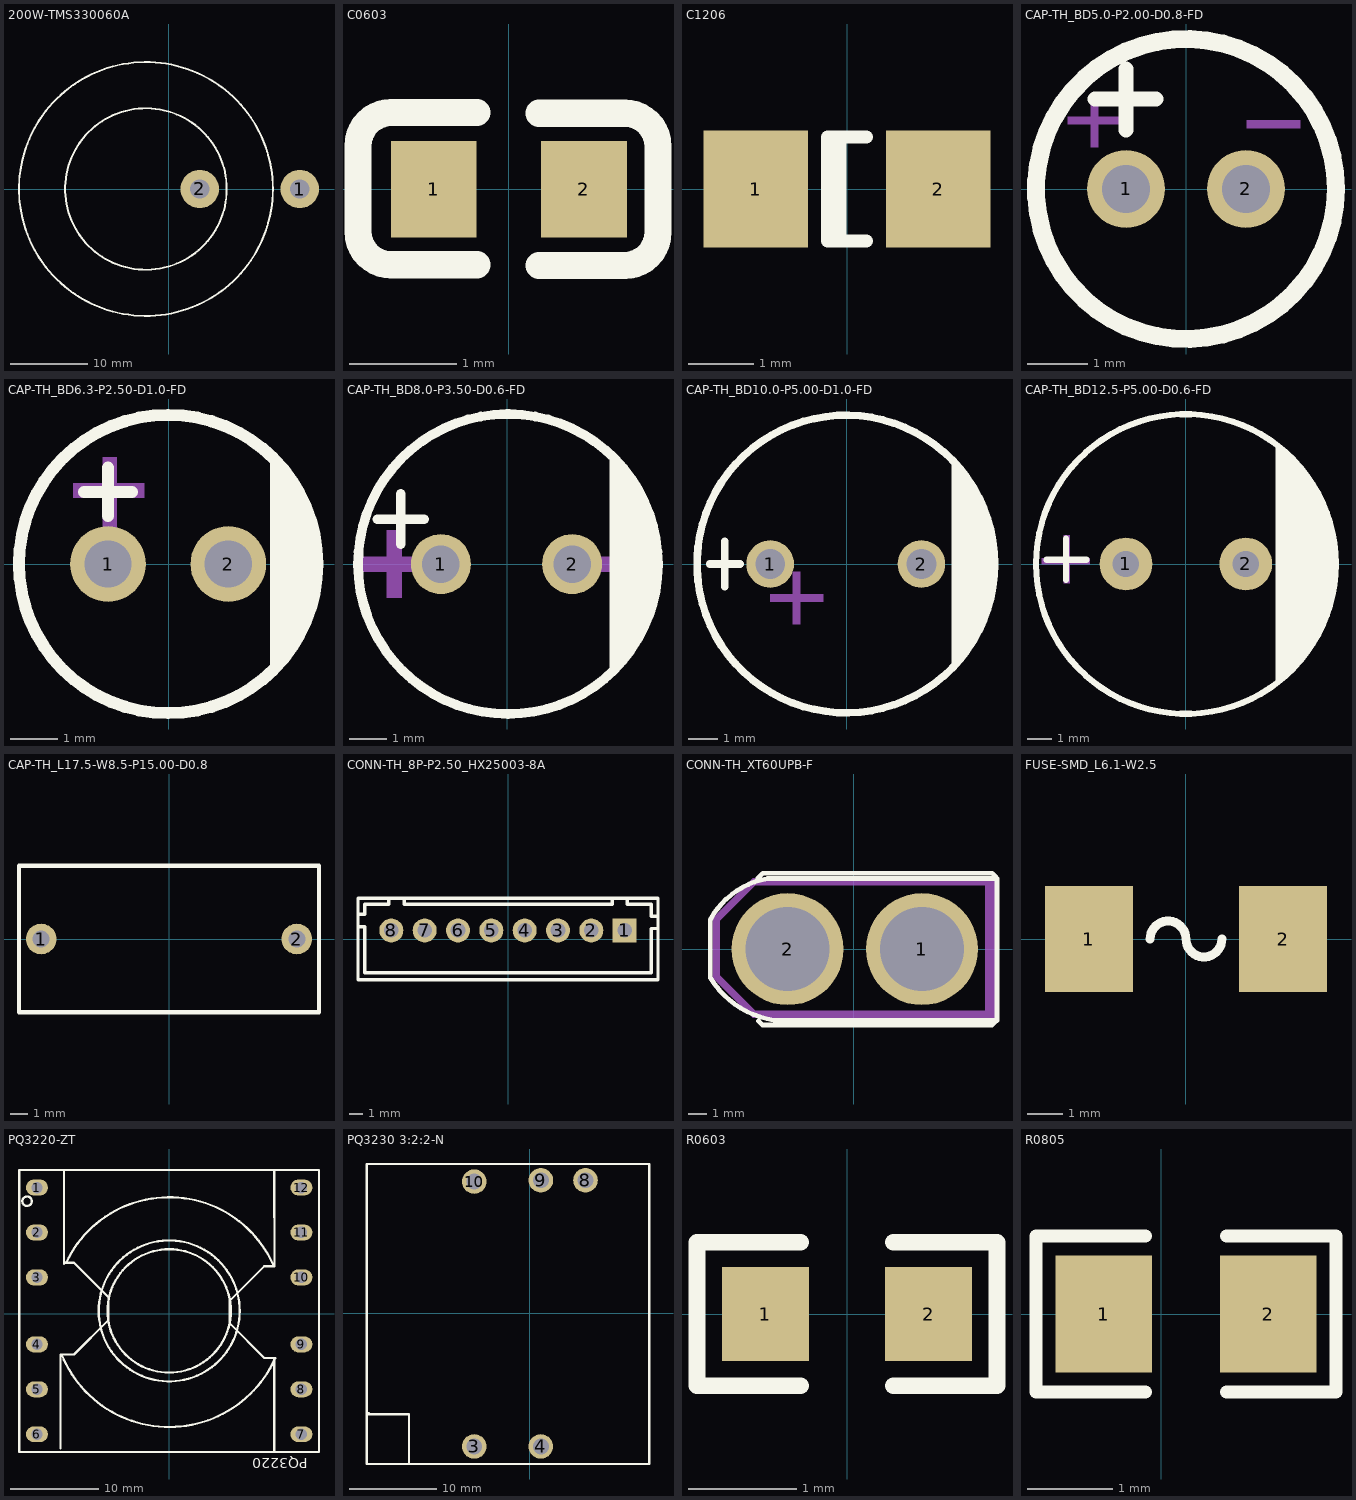
[diagram p0: the footprints below, top view; thin cyan lines are the x and y axes]
# Altium footprint library MISC84449-2.PcbLib: 30 footprints (part 1 of 2)
Each footprint in its own frame and in the unit in brackets; x right, y up, seen from the top. Pads: shape width x height; smd on the part's side, far side on the other; paste and mask are expansions set on the pad; w line width, h text height; cw(c..) or ccw(c..) is an arc to the next point about the centre after c.

## 200W-TMS330060A [mm]
pads (2):
  round 5 hole 2.5: 1(17,0) 2(4,0)
Top Overlay:
  circle w0.254: c-3,0 r16.5
  circle w0.254: c-3,0 r10.5

## C0603 [mm]
pads (2):
  rect 0.8x0.9 smd: 1(-0.7,0) 2(0.7,0)
Top Overlay:
  lines w0.254: -0.296,-0.704 -1.096,-0.704 cw(c-1.096,-0.394) -1.406,-0.394 -1.405,0.406 cw(c-1.096,0.406) -1.096,0.715 -0.296,0.715 ; 0.28,-0.71 1.08,-0.71 ccw(c1.08,-0.4) 1.39,-0.4 1.39,0.4 ccw(c1.08,0.4) 1.08,0.71 0.28,0.71

## C1206 [mm] "Chip Capacitor; Body 3.2 x 1.6 mm (LxW typ)"
height 1.35
pads (2):
  rect 1.6x1.8 smd: 1(-1.4,0) 2(1.4,0)
Top Overlay:
  lines w0.2: -0.11,-0.8 -0.11,0.8 ; 0.3,-0.8 -0.3,-0.8 -0.3,0.8 0.3,0.8

## CAP-TH_BD5.0-P2.00-D0.8-FD [mm]
pads (2):
  round 1.3 hole 0.8: 1(-1,0) 2(1,0)
Top Overlay:
  circle w0.3: c0,0 r2.5
  lines w0.254: -1.516,1.5 -0.5,1.5 ; -1,0.984 -1,2
Mechanical 15:
  region: 1.016,1.143 1.905,1.143 1.905,1.016 1.016,1.016
  region: -1.588,0.699 -1.588,1.587 -1.461,1.587 -1.46,0.699
  region: -1.969,1.206 -1.08,1.206 -1.08,1.079 -1.969,1.079

## CAP-TH_BD6.3-P2.50-D1.0-FD [mm]
pads (2):
  round 1.6 hole 1: 1(-1.28,0) 2(1.26,0)
Top Overlay:
  circle w0.254: c-0.01,0 r3.15
  region: 2.15,2.287 2.27,2.184 2.585,1.816 2.838,1.402 3.023,0.955 3.136,0.483 3.175,0 3.136,-0.483 3.023,-0.955 2.838,-1.402 2.585,-1.816 2.27,-2.184 2.15,-2.287 2.149,-2.286
  lines w0.254: -1.788,1.524 -0.772,1.524 ; -1.28,1.016 -1.28,2.032
Mechanical 15:
  region: -2.01,1.7 -0.51,1.7 -0.51,1.4 -2.01,1.4
  region: -1.391,0.752 -1.391,2.252 -1.091,2.252 -1.091,0.752

## CAP-TH_BD8.0-P3.50-D0.6-FD [mm]
pads (2):
  round 1.6 hole 1: 1(-1.769,-0.001) 2(1.731,-0.001)
Top Overlay:
  region: 2.734,-3.003 3.039,-2.654 3.356,-2.18 3.608,-1.669 3.792,-1.129 3.903,-0.57 3.94,-0.001 3.903,0.568 3.792,1.128 3.608,1.668 3.356,2.179 3.039,2.653 2.734,3.002 2.731,2.999
  lines w0.254: -3.464,1.199 -2.219,1.199 ; -2.841,0.526 -2.841,1.873 ; -0.017,4 ccw(c0.019,0) 0.055,4
Mechanical 15:
  region: -3.219,-0.901 -2.819,-0.901 -2.819,0.899 -3.219,0.899
  region: -3.919,0.199 -3.919,-0.201 -2.119,-0.201 -2.119,0.199
  region: 2.081,0.199 2.081,-0.201 3.881,-0.201 3.881,0.199

## CAP-TH_BD10.0-P5.00-D1.0-FD [mm]
pads (2):
  round 1.6 hole 1: 1(-2.578,0) 2(2.502,0)
Top Overlay:
  circle w0.254: c-0.038,0 r5
  region: 3.518,3.556 3.518,-3.556 4.28,-2.54 4.788,-1.016 5.042,0.508 4.788,1.524
  lines w0.254: -4.61,0 -3.594,0 ; -4.102,-0.762 -4.102,0.762
Mechanical 15:
  region: -1.816,-2.032 -1.562,-2.032 -1.562,-0.254 -1.816,-0.254
  region: -2.578,-1.016 -0.8,-1.016 -0.8,-1.27 -2.578,-1.27

## CAP-TH_BD12.5-P5.00-D0.6-FD [mm]
pads (2):
  round 2.2 hole 1.1: 1(-2.5,0) 2(2.5,0)
Top Overlay:
  circle w0.254: c0,0 r6.25
  region: 3.75,5 3.75,-5 4.482,-4.268 4.489,-4.274 4.941,-3.769 5.333,-3.216 5.661,-2.623 5.92,-1.997 6.108,-1.345 6.221,-0.677 6.259,0 6.221,0.677 6.108,1.345 5.92,1.997 5.661,2.623 5.333,3.216 4.941,3.769 4.489,4.274 4.482,4.268
  lines w0.254: -5.817,0.178 -4.14,0.178 ; -5.004,-0.66 -5.004,1.067
Mechanical 15:
  region: -5.092,-0.811 -5.092,1.189 -4.842,1.189 -4.842,-0.811
  region: -6,0.25 -4,0.25 -4,0 -6,0

## CAP-TH_L17.5-W8.5-P15.00-D0.8 [mm]
pads (2):
  round 1.8 hole 1: 1(-7.5,0) 2(7.5,0)
Top Overlay:
  lines w0.254: -8.8,-4.3 8.8,-4.3 8.8,4.3 -8.8,4.3 -8.8,-4.3

## CONN-TH_8P-P2.50_HX25003-8A [mm]
pads (8):
  rect 1.8x1.8 hole 1.1: 1(8.75,0.646)
  round 1.8 hole 1.1: 2(6.25,0.646) 3(3.75,0.646) 4(1.25,0.646) 5(-1.25,0.646) 6(-3.75,0.646) 7(-6.25,0.646) 8(-8.75,0.646)
Top Overlay:
  lines w0.254: -11.25,0.915 -10.75,0.915 -10.75,-2.521 10.749,-2.521 10.749,0.786 11.249,0.786 ; -11.25,1.845 -10.75,1.845 -10.75,2.604 -8.944,2.604 -8.944,3.054 ; -7.8,2.604 7.8,2.604 ; -7.793,2.601 -7.793,3.05 ; 7.807,2.601 7.807,3.05 ; 8.943,2.604 10.749,2.604 10.749,1.715 11.249,1.715 ; 8.95,2.602 8.95,3.05 ; -11.25,-3.054 11.25,-3.054 11.25,3.046 -11.25,3.046 -11.25,-3.054

## CONN-TH_XT60UPB-F [mm]
pads (2):
  round 6 hole 4.5: 1(3.663,0) 2(-3.536,0)
Top Overlay:
  lines w0.254: -7.683,-1.524 -7.683,1.576 cw(c-3.873,-0.482) -4.625,3.783 7.683,3.783 7.683,-3.819 ; -7.668,-1.548 ccw(c-3.507,1.016) -4.283,-3.81 7.658,-3.81 ; -5.119,3.819 -4.874,4.064 -4.827,4.064 7.419,4.064 7.638,3.844 ; -5.099,-3.844 -4.88,-4.064 7.365,-4.064 7.413,-4.064 7.658,-3.819
Mechanical 15:
  region: -5.397,3.81 -7.556,1.651 -7.303,1.397 -5.143,3.556
  region: -7.556,-1.524 -5.397,-3.683 -5.143,-3.429 -7.302,-1.27
  region: -7.556,1.651 -7.556,-1.524 -7.175,-1.524 -7.175,1.651
  region: -5.397,3.81 7.556,3.81 7.556,3.429 -5.271,3.429
  region: -5.397,-3.683 -5.397,-3.302 7.556,-3.302 7.556,-3.683
  region: 7.556,3.429 7.556,-3.302 7.049,-3.302 7.049,3.429

## FUSE-SMD_L6.1-W2.5 [mm]
pads (2):
  rect 2.5x3 smd: 1(-2.75,0) 2(2.75,0)
Top Overlay:
  lines w0.254: -1.016,0 cw(c-0.508,0) 0,0 ccw(c0.508,0) 1.016,0

## PQ3220-ZT [mm]
pads (12):
  oval 2.5x1.8 hole 1.3: 1(-14.98,14.318) 2(-14.98,9.218) 3(-14.98,4.119) 4(-14.98,-3.481) 5(-14.98,-8.581) 6(-14.98,-13.681) 7(15.02,-13.682) 8(15.02,-8.581) 9(15.02,-3.481) 10(15.02,4.119) 11(15.02,9.218) 12(15.02,14.318)
Top Overlay:
  circle w0.254: c0.02,0.319 r7
  circle w0.254: c0.02,0.319 r8
  circle w0.254: c-16.109,12.765 r0.539
  lines w0.254: -17.02,16.318 17.02,16.318 ; -16.98,-15.681 -16.98,16.318 ; -16.957,-15.681 17.02,-15.681 ; -12.299,-15.302 -12.299,-4.637 ; -11.918,5.78 -10.787,5.78 -6.85,1.843 -6.85,-0.697 -10.787,-4.634 -12.184,-4.634 ccw(c0.02,0.319) 12.044,-5.059 ; -11.903,5.653 -11.903,16.318 ; -11.647,5.83 cw(c0.02,0.319) 11.788,5.614 ; 11.946,-15.681 11.946,-5.015 10.815,-5.015 6.878,-1.078 6.878,1.462 10.815,5.399 11.958,5.399 11.946,16.318 ; 17.02,-15.687 17.02,16.315
  text "PQ3220" at 15.748,-16.383 h1.14

## PQ3230 3:2:2-N [mm]
pads (5):
  round 2.8 hole 1.8: 3(-6.342,-15.17) 4(1.258,-15.17) 8(6.342,15.17) 9(1.262,15.17) 10(-6.342,15.03)
Top Overlay:
  lines w0.254: -18.364,-11.372 -18.364,-11.499 -13.787,-11.499 -13.787,-17.168 -12.141,-17.168 ; -18.59,-17.169 13.61,-17.169 13.61,17.031 -18.59,17.031 -18.59,-17.169

## R0603 [mm]
pads (2):
  rect 0.806x0.864 smd: 1(-0.753,0) 2(0.753,0)
Top Overlay:
  lines w0.152: -0.426,-0.661 -1.385,-0.661 -1.385,0.661 -0.426,0.661 ; 0.426,-0.661 1.385,-0.661 1.385,0.661 0.426,0.661
Top Paste:
  region: -0.355,0.4 -0.355,0.172 -0.735,0.172 -0.735,-0.158 -0.355,-0.158 -0.355,-0.4 -0.405,-0.45 -1.195,-0.45 -1.245,-0.4 -1.245,0.4 -1.195,0.45 -0.405,0.45
  region: 1.195,0.45 0.395,0.45 0.345,0.4 0.345,0.172 0.715,0.172 0.715,-0.158 0.345,-0.158 0.345,-0.4 0.395,-0.45 1.195,-0.45 1.245,-0.4 1.245,0.4

## R0805 [mm]
pads (2):
  rect 1.133x1.377 smd: 1(-0.678,0) 2(1.254,0)
Top Overlay:
  lines w0.152: -0.188,-0.917 -1.473,-0.917 -1.473,0.917 -0.188,0.917 ; 0.764,-0.917 2.049,-0.917 2.049,0.917 0.764,0.917
Top Paste:
  region: 0.738,-0.64 0.738,-0.22 1.183,-0.22 1.183,0.23 0.743,0.23 0.738,0.64 0.788,0.69 1.938,0.69 1.988,0.64 1.988,-0.64 1.938,-0.69 0.788,-0.69
  region: -1.412,-0.64 -1.412,0.64 -1.362,0.69 -0.212,0.69 -0.162,0.64 -0.157,0.23 -0.607,0.23 -0.607,-0.22 -0.167,-0.22 -0.162,-0.64 -0.212,-0.69 -1.362,-0.69